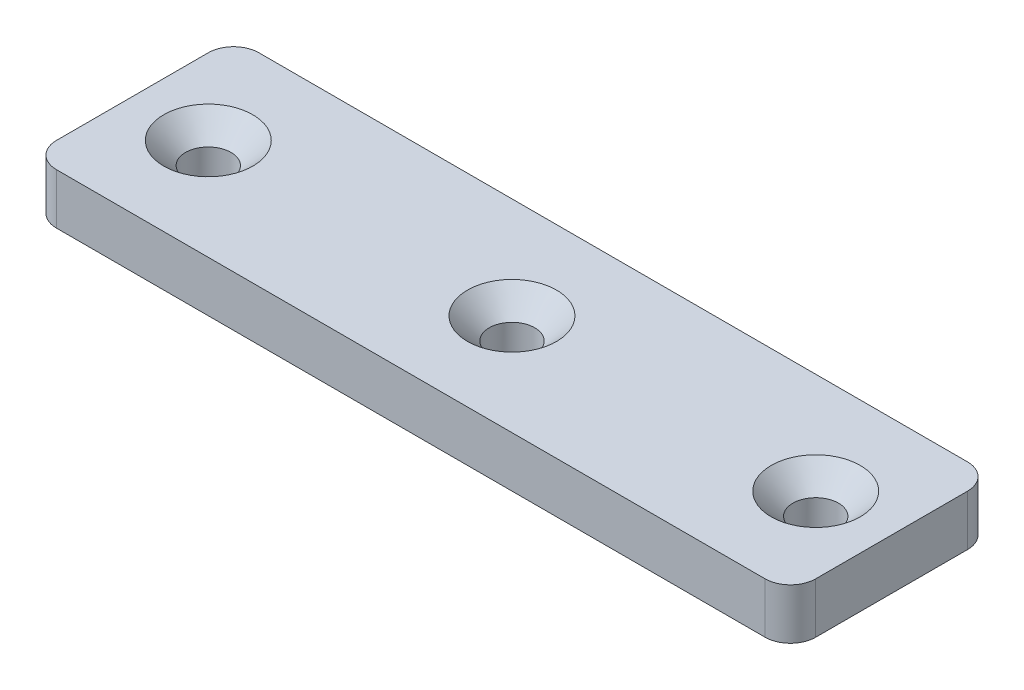
from build123d import *

# Parameters (mm, degrees)
SKETCH1_W                                  = 150
SKETCH1_H                                  = 40
BOSS_EXTRUDE1_DEPTH                        = 10
FILLET1_R                                  = 5
SOCKET_BUTTON_HEAD_SCREW_HOLE1_D           = 9
SOCKET_BUTTON_HEAD_SCREW_HOLE1_DEPTH       = 19.75
SOCKET_BUTTON_HEAD_SCREW_HOLE1_CSINK_D     = 17.6
SOCKET_BUTTON_HEAD_SCREW_HOLE1_CSINK_ANGLE = 90
SOCKET_BUTTON_HEAD_SCREW_HOLE1_TIP         = 2.703872786


with BuildPart() as part:
    # Sketch1 → Boss-Extrude1 (new body)
    with BuildSketch(Plane(origin=(0, 0, 0), x_dir=(1, 0, 0), z_dir=(0, 1, 0))):
        with Locations((75, 20)):
            Rectangle(SKETCH1_W, SKETCH1_H)
    extrude(amount=BOSS_EXTRUDE1_DEPTH)

    # Fillet1
    fillet1_edges = [part.edges().sort_by_distance(p)[0] for p in [
        (0, 5, -40),
        (150, 5, -40),
        (150, 5, 0),
        (0, 5, 0),
    ]]
    fillet(fillet1_edges, radius=FILLET1_R)

    # Socket Button Head Screw Hole1
    with Locations(Plane(origin=(0, 10, 0), x_dir=(1, 0, 0), z_dir=(0, 1, 0))):
        with Locations((75, 20), (15, 20), (135, 20)):
            CounterSinkHole(SOCKET_BUTTON_HEAD_SCREW_HOLE1_D / 2, SOCKET_BUTTON_HEAD_SCREW_HOLE1_CSINK_D / 2, depth=SOCKET_BUTTON_HEAD_SCREW_HOLE1_DEPTH, counter_sink_angle=SOCKET_BUTTON_HEAD_SCREW_HOLE1_CSINK_ANGLE)
            with Locations((0, 0, -(SOCKET_BUTTON_HEAD_SCREW_HOLE1_DEPTH + SOCKET_BUTTON_HEAD_SCREW_HOLE1_TIP / 2))):  # 118° drill point
                Cone(0, SOCKET_BUTTON_HEAD_SCREW_HOLE1_D / 2, SOCKET_BUTTON_HEAD_SCREW_HOLE1_TIP, mode=Mode.SUBTRACT)


solid = part.part
